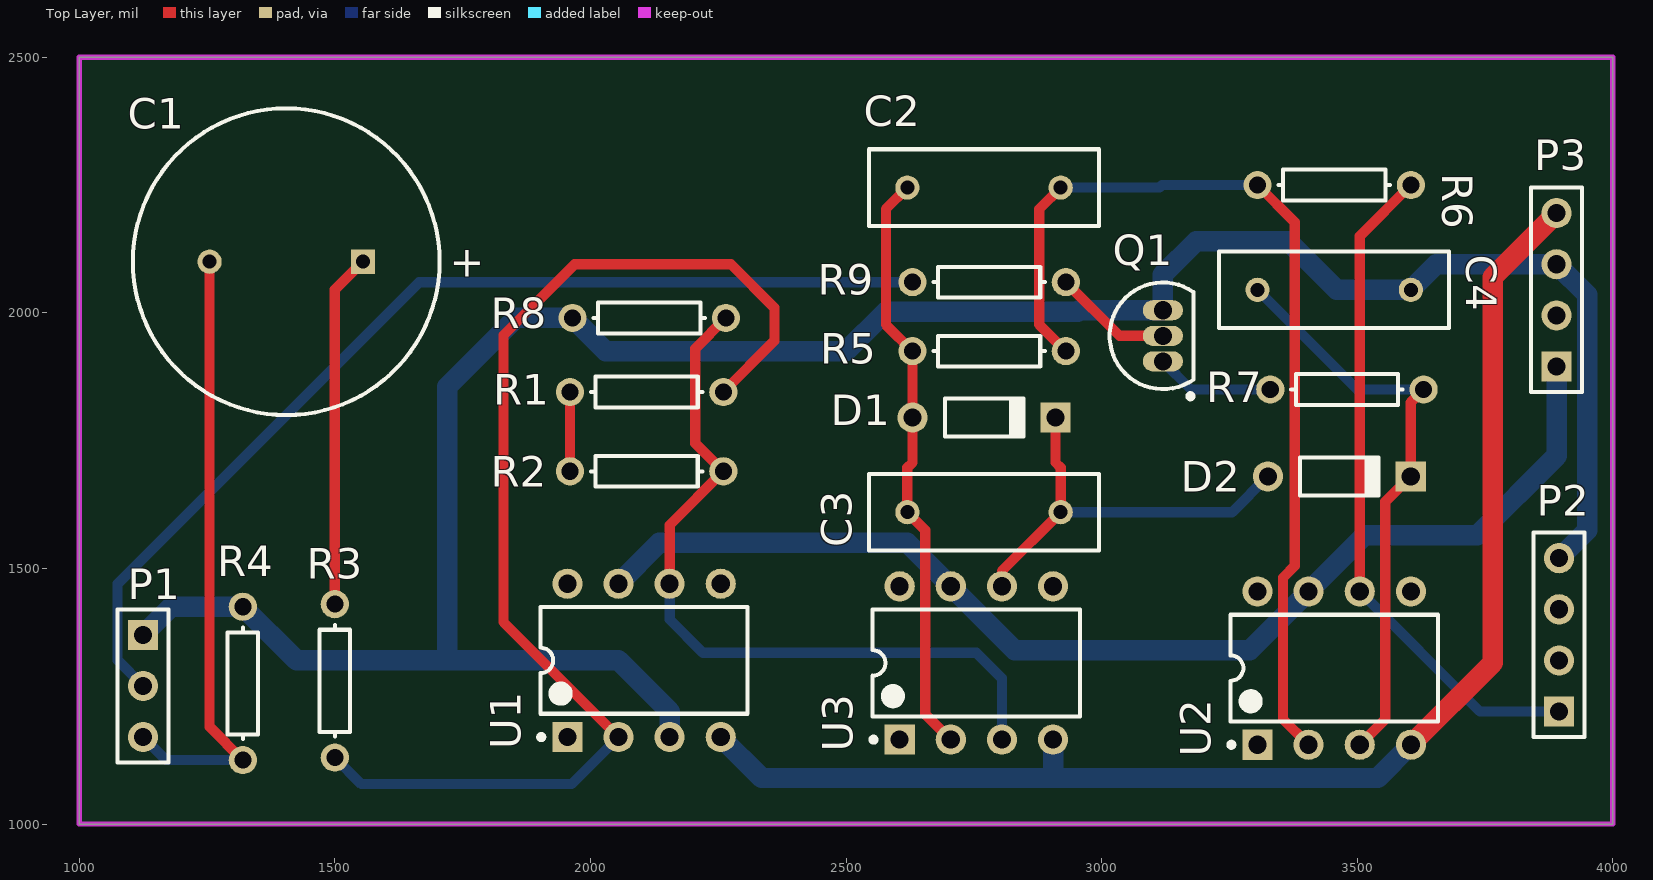
[diagram p0: Top Layer view]
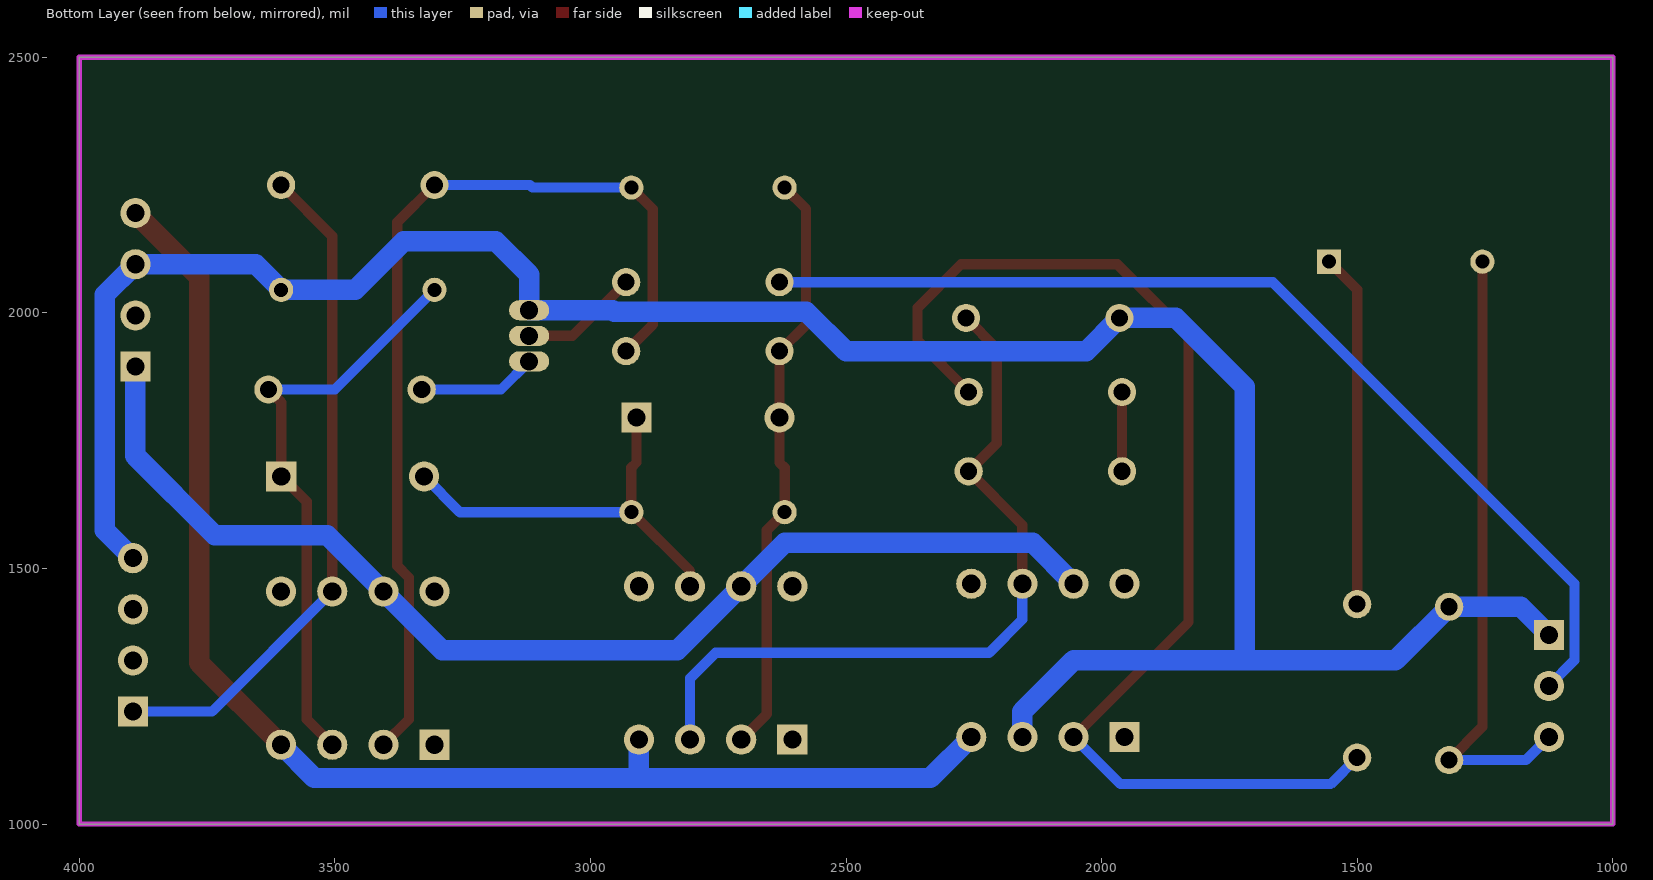
[diagram p1: Bottom Layer view, seen from below]
# Altium PCB MISC80815.PcbDoc
Units mil, origin at the board's own origin, x right, y up, seen from the top; angles counter-clockwise.
Board outline 3000 x 1500 mil, 2 copper layers (Top Layer, Bottom Layer); 22 components, 16 nets, 68 pads, 0 vias.

## Layer stack, top to bottom (the 12.6 mil dielectric is the usual default, probably not edited)
Top Solder: solder mask 0.4, Solder Resist, Dk 3.5
Top Layer: signal copper 1.4
Dielectric 1: dielectric 12.6, FR-4, Dk 4.8
Bottom Layer: signal copper 1.4
Bottom Solder: solder mask 0.4, Solder Resist, Dk 3.5

## Board outline
1000,1000 1000,2500 4000,2500 4000,1000

## Design rules (kind name [scope] priority, off if disabled: settings)
Clearance [All] p1: gap=10
PolygonConnect [All] p1: connectstyle=Relief reliefconductorwidth=10 reliefentries=4 polygonreliefangle="90 Angle" airgapwidth=10
RoutingVias [All] p1: holewidth=28 width=50 viastyle="Through Hole" minholewidth=28 minwidth=50 maxholewidth=28 maxwidth=50
SolderMaskExpansion [All] p1: expansion=4
Width [All] p1: maxlimit=40 minlimit=20 preferedwidth=20
30 further rules are at their usual default settings.

## Classes and differential pairs
component class 子图2: C2 C3 C4 D1 D2 P2 P3 Q1 R5 R6 R7 R8 R9 U2 U3
component class 子图1: C1 P1 R1 R2 R3 R4 U1

## Components (designator, comment, footprint, x,y, rotation, side; value= is the part's Value field where it differs from the comment)
C1 "Cap Pol1" RB7.6-15 1405,2100 r0 top
C2 "Cap" RAD-0.3 2770,2245 r180 top
C3 "Cap" RAD-0.3 2770,1610 r180 top
C4 "Cap" RAD-0.3 3455,2045 r0 top
D1 "Diode 1N914" DO-35 2770,1795 r0 top
D2 "Diode 1N914" DO-35 3465,1680 r0 top
P1 "Header 3" HDR1X3 1125,1370 r270 top
P2 "Header 4" HDR1X4 3895,1220 r90 top
P3 "Header 4" HDR1X4 3890,1895 r90 top
Q1 "NPN" TO-226-AA 3120,1955 r0 top
R1 "Res1" AXIAL-0.3 2110,1845 r180 top
R2 "Res1" AXIAL-0.3 2110,1690 r0 top
R3 "Res1" AXIAL-0.3 1500,1280 r270 top
R4 "Res1" AXIAL-0.3 1320,1275 r270 top
R5 "Res1" AXIAL-0.3 2780,1925 r0 top
R6 "Res1" AXIAL-0.3 3455,2250 r0 top
R7 "Res1" AXIAL-0.3 3480,1850 r180 top
R8 "Res1" AXIAL-0.3 2115,1990 r0 top
R9 "Res1" AXIAL-0.3 2780,2060 r180 top
U1 "UA741AN" DIP-8 2105,1320 r90 top
U2 "UA741AN" DIP-8 3455,1305 r90 top
U3 "UA741AN" DIP-8 2755,1315 r90 top

## Footprints (in the part's own frame and the unit in brackets; to place one, negate y for a bottom-side part, rotate by r counter-clockwise, add the part's x,y. Pads: shape width x height; smd on the part's side, far side on the other; paste and mask are expansions set on the pad)
AXIAL-0.3 [mm] "Axial Device, Thru-Hole; 2 Leads; 0.3 in Pin Spacing"
  round 1.4 hole 0.85: 1(-3.81,0) 2(3.81,0)
  silkscreen extent -2.77,-0.76 2.77,0.76
DIP-8 [mm] "DIP; 8 Leads; Row Spacing 7.62 mm; Pitch 2.54 mm"
  rect 1.5x1.5 hole 0.9: 1(-3.81,3.81)
  round 1.5 hole 0.9: 2(-3.81,1.27) 3(-3.81,-1.27) 4(-3.81,-3.81) 5(3.81,-3.81) 6(3.81,-1.27) 7(3.81,1.27) 8(3.81,3.81)
  silkscreen extent -3.93,-5.15 2.65,5.23, body extent -3.6,-5.15 3.6,5.15, height 5.08
DO-35 [mm] "Diode, Axial; Body 3.8 x 1.9 mm (LxDia. max), Lead Dia. 0.53 mm (max)"
  round 1.5 hole 0.9: 1(-3.55,0)
  rect 1.5x1.5 hole 0.9: 2(3.55,0)
  silkscreen extent -1.95,-0.95 2.05,0.95
HDR1X3 [mm] "Connector; Header; 3 Position"
  rect 1.5x1.5 hole 0.9: 1(0,0)
  round 1.5 hole 0.9: 2(2.54,0) 3(5.08,0)
  silkscreen extent -1.27,-1.27 6.35,1.27
HDR1X4 [mm] "Connector; Header; 4 Position"
  rect 1.5x1.5 hole 0.9: 1(0,0)
  round 1.5 hole 0.9: 2(2.54,0) 3(5.08,0) 4(7.62,0)
  silkscreen extent -1.27,-1.27 8.89,1.27
RAD-0.3 [mm] "Radial Cap, Thru-Hole; 2 Leads; 0.3 in Pin Spacing"
  round 1.2 hole 0.7: 1(-3.81,0) 2(3.81,0)
  silkscreen extent -5.71,-1.91 5.71,1.91
RB7.6-15 [mm] "Polarized Capacitor (Radial); 2 Leads"
  rect 1.2x1.2 hole 0.7: 1(3.81,0)
  round 1.2 hole 0.7: 2(-3.81,0)
  silkscreen extent -7.62,-7.62 7.62,7.62
TO-226-AA [mm] "TO, Flat Index; 3 In-Line, Axial Leads; Body Dia. 4.8mm; Leads 0.55 x 0.51 mm (max)"
  oval 2x1 hole 0.9: 1(0,-1.27) 2(0,0) 3(0,1.27)
  silkscreen extent -2.65,-3.13 1.52,2.65, body extent -2.65,-2.66 1.52,2.66, height 5.33

## Part data
C1: "Polarized Capacitor (Radial)"
C2 C3 C4: "Capacitor"
D1 D2: "High Conductance Fast Diode"
P1: "Header, 3-Pin"
P2 P3: "Header, 4-Pin"
Q1: "NPN Bipolar Transistor"
R1 R2 R3 R4 R5 R6 R7 R8 R9: "Resistor"
U1 U2 U3: "General-Purpose Single Operational Amplifier"

## Nets (pads, with @x,y where several pads share a name; then routed paths per layer and width w, separated by ;. In a path a pad name is that pad's centre, name@x,y a point inside that pad or via, vN(x,y) a via of type N, cw(c..) or ccw(c..) an arc to the next point about the centre after c; other vN are vias at no path point)
GND: C4.2 P1.1 P2.4 P3.3 Q1.3 R4.1 R8.1 U1.3 | length 4788.3
  Bottom Layer w40: P1.1 1180,1425 R4.1 1425,1320 1720,1320 ; U1.3 2155,1220 2055,1320 1720,1320 ; P2.4 3950,1575 3950,2035 P3.3 3655,2095 C4.2 3460,2045 3365,2140 3185,2140 3120,2075 Q1.3 2956.4,2005 2953.84,2002.44 2577.44,2002.44 2500,1925 2030,1925 R8.1 1855,1990 1720,1855 1720,1320
NetC1_1: C1.1 R3.1 | length 692.8
  Top Layer w20: R3.1 1500,2045 C1.1
NetC1_2: C1.2 P1.3 R4.2 | length 1215.6
  Top Layer w20: C1.2 1255,1190 R4.2
  Bottom Layer w20: P1.3 1170,1125 R4.2
NetC2_1: C2.1 R5.2 R6.1 U2.2 | length 1901.5
  Top Layer w20: C2.1 2878,2203 2878,1977 R5.2 ; R6.1 3378,2177 3378,1505 3355,1482 3355,1205 U2.2
  Bottom Layer w20: C2.1 3113,2245 3118,2250 R6.1
NetC2_2: C2.2 C3.2 D1.1 R5.1 U3.2 | length 1158.5
  Top Layer w20: C2.2 2578,2203 2578,1977 R5.1 2630,1859.24 2630.24,1859 D1.1 2630.24,1707.24 2620,1697 C3.2 2655,1575 2655,1215 U3.2
NetC3_1: C3.1 D1.2 D2.1 U3.6 | length 816.1
  Top Layer w20: U3.6 2805,1495 C3.1 2920,1697 2909.76,1707.24 D1.2
  Bottom Layer w20: C3.1 3255.24,1610 D2.1
NetC4_1: C4.1 D2.2 R7.1 U2.3 | length 1152.5
  Top Layer w20: U2.3 3555,1205 3555,1630.24 D2.2 3604.76,1824.76 R7.1
  Bottom Layer w20: C4.1 3500,1850 R7.1
NetP1_2: P1.2 R9.2 | length 2020.1
  Bottom Layer w20: P1.2 1075,1320 1075,1470 1665,2060 R9.2
NetP2_1: P2.1 R6.2 U2.6 | length 1323.8
  Top Layer w20: U2.6 3505,2150 R6.2
  Bottom Layer w20: U2.6 3740,1220 P2.1
NetQ1_1: Q1.1 R7.2 | length 232.8
  Bottom Layer w20: Q1.1 3175,1850 R7.2
NetQ1_2: Q1.2 R9.1 | length 233.5
  Top Layer w20: R9.1 3035,1955 Q1.2
NetR1_1: R1.1 R3.2 U1.2 | length 2323
  Top Layer w20: U1.2 1830,1395 1830,1956 1969,2095 2275,2095 2360,2010 2360,1945 R1.1
  Bottom Layer w20: R3.2 1552,1078 1963,1078 U1.2
NetR1_2: R1.2 R2.1 | length 155
  Top Layer w20: R2.1 R1.2
NetR2_2: R2.2 R8.2 U1.6 U3.3 | length 1498.8
  Top Layer w20: U1.6 2155,1585 R2.2 2205,1745 2205,1930 R8.2
  Bottom Layer w20: U1.6 2155,1400 2220,1335 2755,1335 2805,1285 U3.3
VCC5: P3.1 U1.7 U2.7 U3.7 | length 2287.5
  Bottom Layer w40: U1.7 2135,1550 2620,1550 U3.7 2830,1340 3290,1340 U2.7 3515,1565 3735,1565 3890,1720 P3.1
VSSM5: P3.4 U1.4 U2.4 U3.4 | length 2643.1
  Top Layer w40: U2.4 3765,1315 3765,2070 P3.4
  Bottom Layer w40: U1.4 2335,1090 2905,1090 ; U3.4 2905,1090 ; U2.4 3540,1090 2905,1090
pads on no net: P2.2 P2.3 P3.2 U1.1 U1.5 U1.8 U2.1 U2.5 U2.8 U3.1 U3.5 U3.8

## Keep-outs
Keep-Out Layer:
  the board outline again, w10